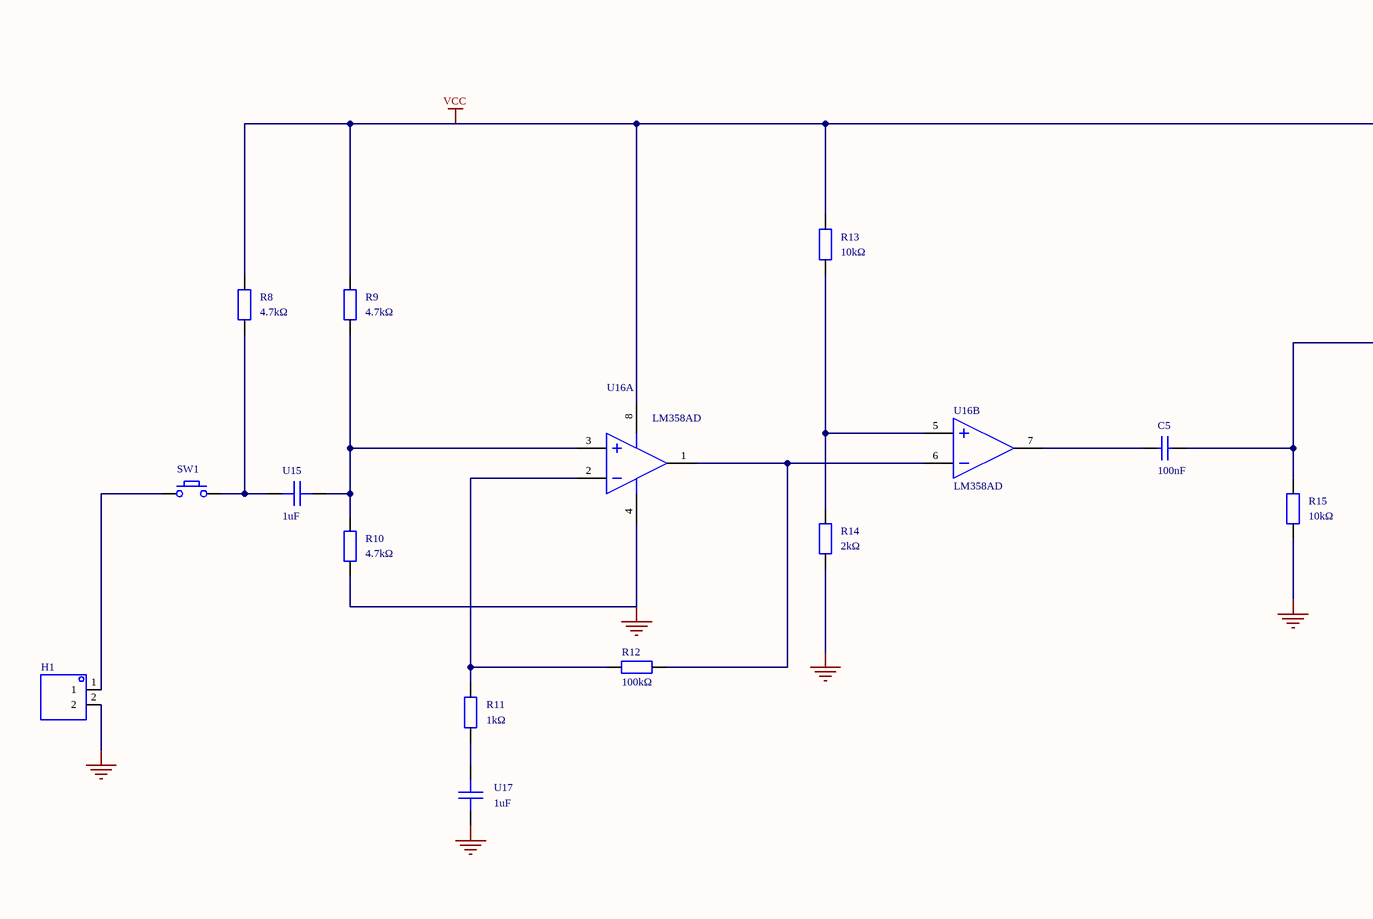
[diagram p0: MISC51104-3.schdoc, left]
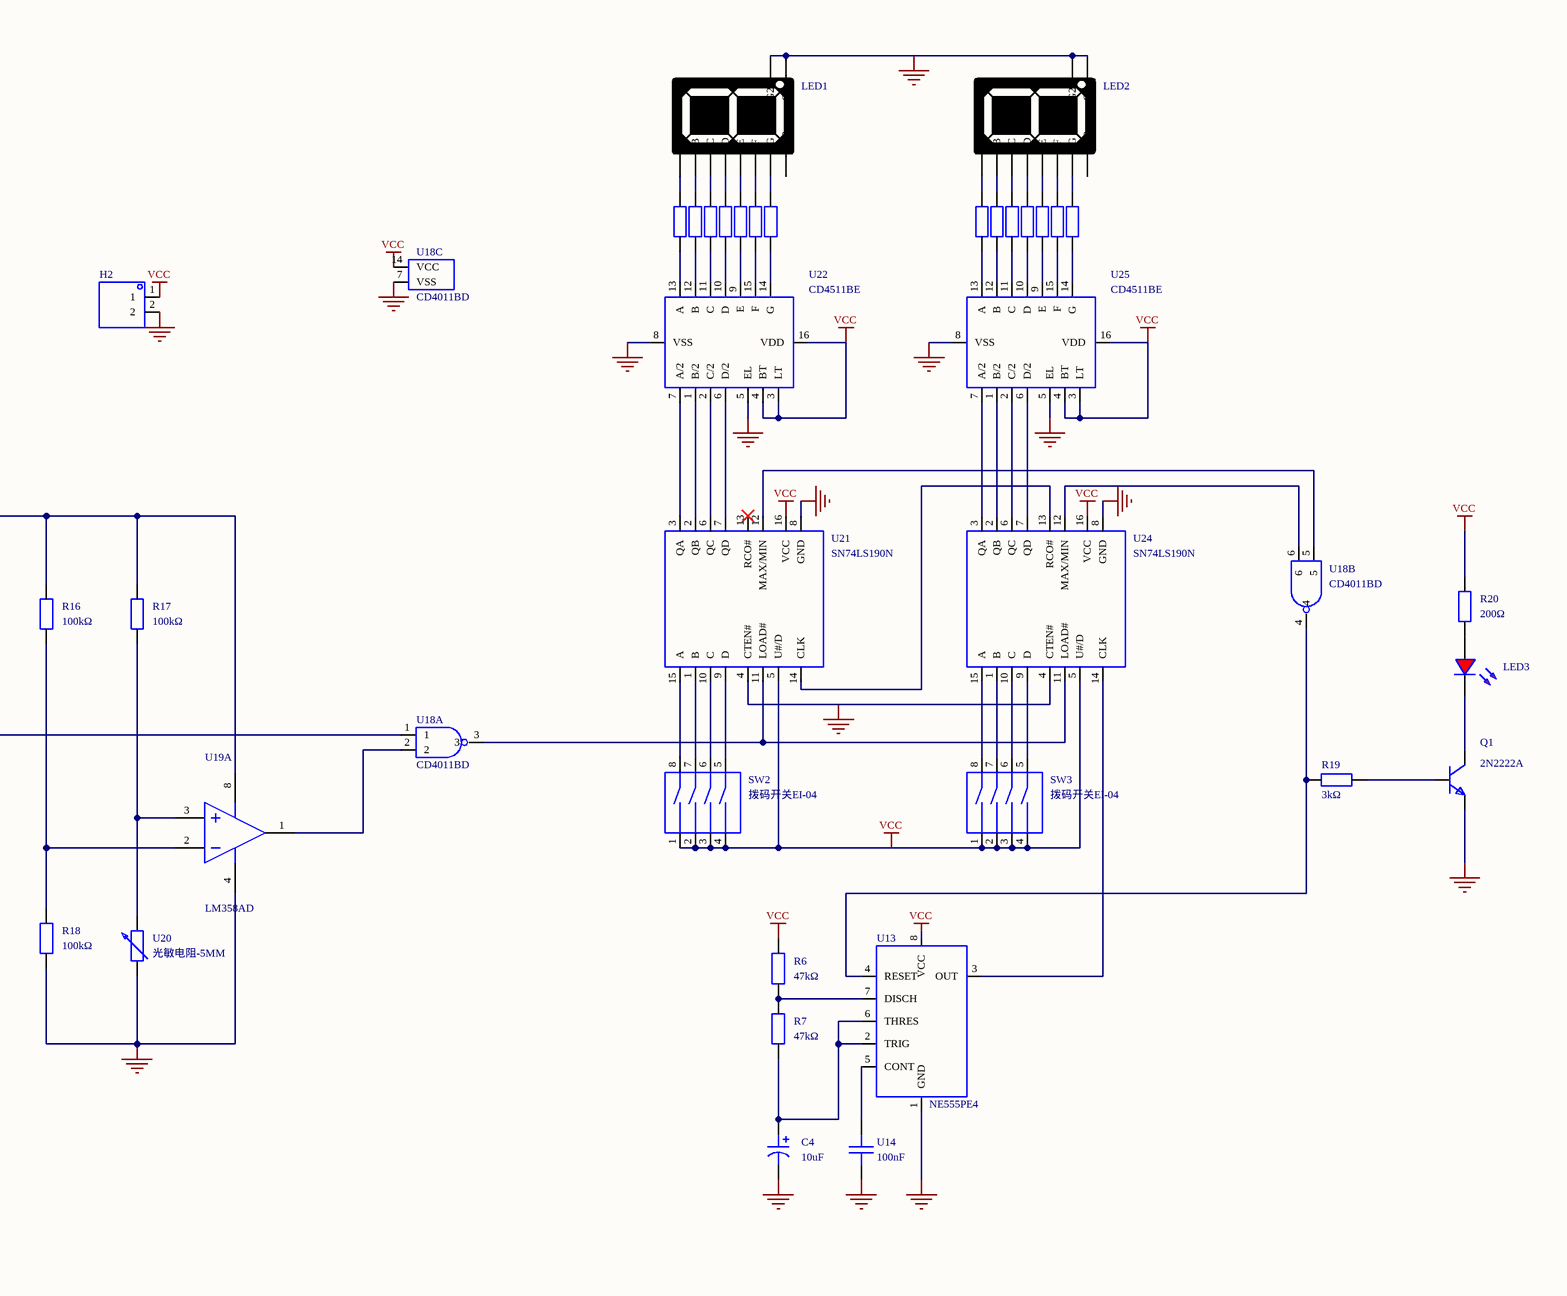
[diagram p1: MISC51104-3.schdoc, right]
# Altium project MISC51104-2.PrjPcb
1 sheet, 52 parts. Net scope: global (net labels, ports and power ports of the same name join across sheets).
Board file: MISC51104.pcbdoc

## Sheet MISC51104-3.schdoc
size 594 x 419 mm; Version: V1.0; @Project Name: MISC51104; @Page Count: 1; @Update Date: 2025-06-07; @Create Date: 2025-06-07; @Schematic Name: MISC51104; @Page No: 1; @Create Time: 21:33:00; @Update Time: 12:58:40; @Board Name: MISC51104

### Parts
C4  10uF  [CAP-TH_BD5.0-P2.00-D0.5-FD]
C5  100nF  [CAP-TH_L4.0-W2.5-P2.50-D0.5-A]
H1  (no value)  [HDR-TH_2P-P2.54-V-M-1]
H2  (no value)  [HDR-TH_2P-P2.54-V-M-1]
LED1  (no value)  [LED-SEG-TH_10P-L12.6-W19.0-P2.54-S15.24-BL]
LED2  (no value)  [LED-SEG-TH_10P-L12.6-W19.0-P2.54-S15.24-BL]
LED3  (no value)  [LED_TH-3mm]
Q1  2N2222A  [TO-92-3_L4.9-W3.7-P1.27-L]
R6  47kΩ  [Res_1/8W]
R7  47kΩ  [Res_1/8W]
R8  4.7kΩ  [Res_1/8W]
R9  4.7kΩ  [Res_1/8W]
R10  4.7kΩ  [Res_1/8W]
R11  1kΩ  [Res_1/8W]
R12  100kΩ  [Res_1/8W]
R13  10kΩ  [Res_1/8W]
R14  2kΩ  [Res_1/8W]
R15  10kΩ  [Res_1/8W]
R16  100kΩ  [Res_1/8W]
R17  100kΩ  [Res_1/8W]
R18  100kΩ  [Res_1/8W]
R19  3kΩ  [Res_1/8W]
R20  200Ω  [Res_1/8W]
R21  10kΩ  [Res_1/8W]  (value not drawn)
R22  10kΩ  [Res_1/8W]  (value not drawn)
R23  10kΩ  [Res_1/8W]  (value not drawn)
R24  10kΩ  [Res_1/8W]  (value not drawn)
R25  10kΩ  [Res_1/8W]  (value not drawn)
R26  10kΩ  [Res_1/8W]  (value not drawn)
R27  10kΩ  [Res_1/8W]  (value not drawn)
R28  10kΩ  [Res_1/8W]  (value not drawn)
R29  10kΩ  [Res_1/8W]  (value not drawn)
R30  10kΩ  [Res_1/8W]  (value not drawn)
R31  10kΩ  [Res_1/8W]  (value not drawn)
R32  10kΩ  [Res_1/8W]  (value not drawn)
R33  10kΩ  [Res_1/8W]  (value not drawn)
R34  10kΩ  [Res_1/8W]  (value not drawn)
SW1  (no value)  [Key_TH_3.5x6x4.3]
SW2  拨码开关EI-04  [SW-TH_DIPSWITCHEI-04]
SW3  拨码开关EI-04  [SW-TH_DIPSWITCHEI-04]
U13  NE555PE4  [PDIP-8_L9.6-W6.4-P2.54-LS7.9-BL-1]
U14  100nF  [CAP-TH_L4.5-W3.0-P2.50-D0.5]
U15  1uF  [CAP-TH_L4.0-W2.5-P2.50-D0.5]
U16  LM358AD  [SOP-8_L4.9-W3.9-P1.27-LS6.0-BL]  (parts A,B of 2)
U17  1uF  [CAP-TH_L4.0-W2.5-P2.50-D0.5]
U18  CD4011BD  [PDIP-14_L19.3-W6.4-P2.54-LS7.9-BL-1]  (parts A,B,C of 3)
U19  LM358AD  [SOP-8_L4.9-W3.9-P1.27-LS6.0-BL]  (part A of 2)
U20  光敏电阻-5MM  [RES-TH_L4.9-W4.3-P3.4]
U21  SN74LS190N  [PDIP-16_L19.2-W6.6-P2.54-LS7.6-BL]
U22  CD4511BE  [DIP-16_L19.8-W6.5-P2.54-LS7.6-BL]
U24  SN74LS190N  [PDIP-16_L19.2-W6.6-P2.54-LS7.6-BL]
U25  CD4511BE  [DIP-16_L19.8-W6.5-P2.54-LS7.6-BL]

### Nets
GND: C4.2 H1.2 H2.2 LED1.3(G1) LED1.8(G2) LED2.3(G1) LED2.8(G2) Q1.1(E) R10.1 R14.1 R15.1 R18.1 U13.1(GND) U14.1 U16.4(VEE) U17.1 U18.7(VSS) U19.4(VEE) U20.1 U21.4(CTEN#) U21.8(GND) U22.5(EL) U22.8(VSS) U24.4(CTEN#) U24.8(GND) U25.5(EL) U25.8(VSS)
VCC: H2.1 R6.2 R8.2 R9.2 R13.2 R16.2 R17.2 R20.2 SW2.1 SW2.2 SW2.3 SW2.4 SW3.1 SW3.2 SW3.3 SW3.4 U13.8(VCC) U16.8(VCC) U18.14(VCC) U19.8(VCC) U21.5(U#/D) U21.16(VCC) U22.3(LT) U22.4(BT) U22.16(VDD) U24.5(U#/D) U24.16(VCC) U25.3(LT) U25.4(BT) U25.16(VDD)
NetC4_1: C4.1 R7.1 U13.2(TRIG) U13.6(THRES)
NetC5_1: C5.1 U16.7(OUT2)
NetC5_2: C5.2 R15.2 U18.1
NetH1_1: H1.1 SW1.A
NetLED1_1: LED1.1(E) R25.2
NetLED1_2: LED1.2(D) R24.2
NetLED1_4: LED1.4(C) R23.2
NetLED1_6: LED1.6(B) R22.2
NetLED1_7: LED1.7(A) R21.2
NetLED1_9: LED1.9(F) R26.2
NetLED1_10: LED1.10(G) R27.2
NetLED2_1: LED2.1(E) R32.2
NetLED2_2: LED2.2(D) R31.2
NetLED2_4: LED2.4(C) R30.2
NetLED2_6: LED2.6(B) R29.2
NetLED2_7: LED2.7(A) R28.2
NetLED2_9: LED2.9(F) R33.2
NetLED2_10: LED2.10(G) R34.2
NetLED3_1: LED3.1(C) R20.1
NetLED3_2: LED3.2(A) Q1.3(C)
NetQ1_2: Q1.2(B) R19.1
NetR6_1: R6.1 R7.2 U13.7(DISCH)
NetR8_1: R8.1 SW1.B U15.1
NetR9_1: R9.1 R10.2 U15.2 U16.3(IN1-)
NetR11_1: R11.1 U17.2
NetR11_2: R11.2 R12.1 U16.2(IN1+)
NetR12_2: R12.2 U16.1(OUT1) U16.6(IN2-)
NetR13_1: R13.1 R14.2 U16.5(IN2+)
NetR16_1: R16.1 R18.2 U19.2(IN1+)
NetR17_1: R17.1 U19.3(IN1-) U20.2
NetR19_2: R19.2 U13.4(RESET) U18.4
NetR21_1: R21.1 U22.13(A)
NetR22_1: R22.1 U22.12(B)
NetR23_1: R23.1 U22.11(C)
NetR24_1: R24.1 U22.10(D)
NetR25_1: R25.1 U22.9(E)
NetR26_1: R26.1 U22.15(F)
NetR27_1: R27.1 U22.14(G)
NetR28_1: R28.1 U25.13(A)
NetR29_1: R29.1 U25.12(B)
NetR30_1: R30.1 U25.11(C)
NetR31_1: R31.1 U25.10(D)
NetR32_1: R32.1 U25.9(E)
NetR33_1: R33.1 U25.15(F)
NetR34_1: R34.1 U25.14(G)
NetSW2_5: SW2.5 U21.9(D)
NetSW2_6: SW2.6 U21.10(C)
NetSW2_7: SW2.7 U21.1(B)
NetSW2_8: SW2.8 U21.15(A)
NetSW3_5: SW3.5 U24.9(D)
NetSW3_6: SW3.6 U24.10(C)
NetSW3_7: SW3.7 U24.1(B)
NetSW3_8: SW3.8 U24.15(A)
NetU13_3: U13.3(OUT) U24.14(CLK)
NetU13_5: U13.5(CONT) U14.2
NetU18_2: U18.2 U19.1(OUT1)
NetU18_3: U18.3 U21.11(LOAD#) U24.11(LOAD#)
NetU18_5: U18.5 U21.12(MAX/MIN)
NetU18_6: U18.6 U24.12(MAX/MIN)
NetU21_2: U21.2(QB) U22.1(B/2)
NetU21_3: U21.3(QA) U22.7(A/2)
NetU21_6: U21.6(QC) U22.2(C/2)
NetU21_7: U21.7(QD) U22.6(D/2)
NetU21_14: U21.14(CLK) U24.13(RCO#)
NetU24_2: U24.2(QB) U25.1(B/2)
NetU24_3: U24.3(QA) U25.7(A/2)
NetU24_6: U24.6(QC) U25.2(C/2)
NetU24_7: U24.7(QD) U25.6(D/2)

Not connected (* = marked no-connect by the designer): LED1 5(DP); LED2 5(DP); U21 13(RCO#)*

### Notes on the sheet
- 2025-06-07
- 原理图
- P1
- 版本
- 尺寸
- A4
- 页    1    共    1

### Library data of the parts
C4 = SHG63V10UF03EC0822: 容值:10uF;精度:±20%;额定电压:63V;; AddInBom: yes; ModelId: aba3b94bdab6406eb4f45c9c765c730e; ModelTransform: 196.85,196.517,0,0,0,0,0,0,-196.85; Tolerance: ±20%; Voltage Rating: 63V; Symbol: SHG63V10UF03EC0822; Device: SHG63V10UF03EC0822; LCSC Part Name: 停产 10uF ±20% 63V; SupplierPart: C5263880; ManufacturerPart: SHG63V10UF03EC0822; Supplier Footprint: 插件,D5xL11mm; JLCPCB Part Class: 扩展库; Datasheet: https://atta.szlcsc.com/upload/public/pdf/source/20221206/74D9A2C5191757C58A566DD8357A6A8B.pdf; Supplier: LCSC; ConvertToPcb: yes; FootprintName: CAP-TH_BD5.0-P2.00-D0.5-FD; ModelName: CAP-TH_BD5.0-P2.00-D0.5-FD; Value: 10uF; Diameter: 5mm; Height - Seated (Max): 11mm
C5 = FA18X7R1H104KNU00: 容值:100nF;精度:±10%;额定电压:50V;温度系数:X7R;; Manufacturer: TDK; AddInBom: yes; ModelId: 286ce451e059442e92b487a621b9c1b6; ModelTransform: 217.63405,98.8187,0,0,0,0,0,0,-196.85; Tolerance: ±10%; Voltage Rated: 50V; Temperature Coefficient: X7R; Symbol: FA18X7R1H104KNU00; Device: FA18X7R1H104KNU00; LCSC Part Name: 100nF ±10% 50V; SupplierPart: C1622804; ManufacturerPart: FA18X7R1H104KNU00; Supplier Footprint: 插件; JLCPCB Part Class: 扩展库; Datasheet: https://atta.szlcsc.com/upload/public/pdf/source/20210607/0A2A90FBDDBAB681A19577D378B4B30C.pdf; Supplier: LCSC; ConvertToPcb: yes; FootprintName: CAP-TH_L4.0-W2.5-P2.50-D0.5-A; ModelName: CAP-TH_L4.0-W2.5-P2.50-D0.5-A; Value: 100nF
H1 H2 = HDR-M_2.54_1x2P: Symbol: 210S-1*2P L=11.6MMGold-plated black; ConvertToPcb: yes; ModelId: 79b2e9f2d70a4d68a1b7098f27c6d4c5; ModelName: HDR-M-2.54_1x2; ModelTransform: 200,100,0,0,0,0,0,0,-118.11; Device: HDR-M_2.54_1x2P; AddInBom: yes; SupplierPart: C124375; Supplier Footprint: 插件; FootprintName: HDR-TH_2P-P2.54-V-M-1
LED1 LED2 = LED_SEG_TH_0.56x1: Symbol: LED_SEG_TH_0.56*1; ConvertToPcb: yes; ModelId: 16c3aae6d39e4ecc9e744d6eeac8d57b; ModelName: LED-SEG-TH_0.56_1p; ModelTransform: 496.062,748.03,0,0,0,0,0,0,-137.795; Device: LED_SEG_TH_0.56x1; AddInBom: yes; Supplier Footprint: 插件; FootprintName: LED-SEG-TH_10P-L12.6-W19.0-P2.54-S15.24-BL
LED3 = LED_TH-R_3mm: ConvertToPcb: yes; ModelId: a497c992633541038a38947cdc58012f; ModelName: LED-TH-3mm_R; ModelTransform: 141.274,153.327,0,0,0,0,-5.984,0,-137.795; Symbol: LED_TH-R; Device: LED_TH-R_3mm; AddInBom: yes; FootprintName: LED_TH-3mm; Supplier Footprint: 插件
Q1 = 2N2222A: 晶体管类型:NPN;集电极电流(Ic):600mA;集射极击穿电压(Vceo):40V;功率(Pd):625mW;直流电流增益(hFE@Ic,Vce):40@500mA,10V;; Manufacturer: ST(先科); Symbol: 2N2222; AddInBom: yes; ModelId: db569d051dcd4484acf2f9e50678fca3; ModelTransform: 180.7872,141.4455,0,0,0,0,0,22.677,-196.85; Transistor Type: NPN; Collector Current (Ic): 600mA; Collector-Emitter Breakdown Voltage (Vceo): 40V; Power Dissipation (Pd): 625mW; Transition Frequency (fT): 250MHz; Collector Cut-Off Current (Icbo): 10nA; Collector-Emitter Saturation Voltage (VCE(sat)@Ic,Ib): 1V@500mA,50mA; Device: 2N2222A; LCSC Part Name: NPN 电流:600mA 耐压:40V; SupplierPart: C118536; ManufacturerPart: 2N2222A; Supplier Footprint: TO-92-3; Datasheet: https://atta.szlcsc.com/upload/public/pdf/source/20170719/C118536_1500457734789828244.pdf; Supplier: LCSC; ConvertToPcb: yes; FootprintName: TO-92-3_L4.9-W3.7-P1.27-L; ModelName: TO-92-3_L4.9-W3.7-P1.27-L; DC Current Gain (hFE@Ic,Vce): 40@500mA,10V; Operating Temperature: -
R6-R34 = Res_AXIAL-1/8W: ConvertToPcb: yes; SymbolName: 电阻; ModelId: b2b5ae7ae4c642178fe0039925c86a3f; ModelName: RES-TH_BD1.8-L3.2-P7.20-D0.4; ModelTransform: 282.86,66.88,253.09,0,0,0,0,0,-191; Device: Res_AXIAL-1/8W; AddInBom: yes; Supplier Footprint: 轴向引线; FootprintName: Res_1/8W
  R6 R7: Value: 47kΩ
  R8-R10: Value: 4.7kΩ
  R11: Value: 1kΩ
  R12 R16-R18: Value: 100kΩ
  R13 R15 R21-R34: Value: 10kΩ
  R14: Value: 2kΩ
  R19: Value: 3kΩ
  R20: Value: 200Ω
SW1 = Key_TH_3.5x6x4.3: ConvertToPcb: yes; ModelId: c3523f9014d949d7ba5445190a3178990819f05c4eef4c71ace90d822a990e87; ModelName: SW-TH_L6.0-W3.5-H5.0-P6.5; ModelTransform: 308.49,137.8,335.08,0,0,0,0,0,-129.92; Device: Key_TH_3.5x6x4.3; AddInBom: yes; Supplier Footprint: 插件; SymbolName: Key_TH_3.5x6x4.3; FootprintName: Key_TH_3.5x6x4.3
SW2 SW3 = 拨码开关EI-04: 类型:平拨,凸起式;电路结构:单刀单掷;开关位数:4位;使用寿命:-;颜色:黑色;; Manufacturer: 圜达; Symbol: DIP switchEI-04; AddInBom: yes; ModelId: 05004328256048a2b98ea2194ea80753; ModelName: SW-TH_DIPSWITCHEI-04-L10.1-W6.0-H3.4-P2.54-LS7.6; ModelTransform: 396.0622,309.842,0,0,0,0,0,0,-137.795; Circuit: 单刀单掷; Number of Positions: 4位; Device: 拨码开关EI-04; LCSC Part Name: 拨码开关EI-04; SupplierPart: C99987; ManufacturerPart: 拨码开关EI-04; Supplier Footprint: -; JLCPCB Part Class: 扩展库; Datasheet: https://atta.szlcsc.com/upload/public/pdf/source/20170504/1493892386551.pdf; Supplier: LCSC; ConvertToPcb: yes; FootprintName: SW-TH_DIPSWITCHEI-04; Type: 平拨,凸起式; Lead Pitch: 2.54mm; Operating Life: -; Color: 黑色
U13 = NE555PE4: 单精度计时器 8-PDIP 0 to 70; Manufacturer: TI(德州仪器); AddInBom: yes; ModelId: 1b8eaf096e7944deafe216467068c10e; ModelTransform: 377.952,318.897,0,0,0,0,0,0,-118.11; Symbol: NE555PE4; Device: NE555PE4; LCSC Part Name: NE555PE4; SupplierPart: C2859604; ManufacturerPart: NE555PE4; Supplier Footprint: PDIP-8; Datasheet: https://www.ti.com/cn/lit/gpn/sa555; Supplier: LCSC; ConvertToPcb: yes; FootprintName: PDIP-8_L9.6-W6.4-P2.54-LS7.9-BL-1; ModelName: PDIP-8_L9.6-W6.4-P2.54-LS7.9-BL-1
U14 = FA14X8R1H104KNU00: 容值:100nF;精度:±10%;额定电压:50V;温度系数:X8R;; Manufacturer: TDK; AddInBom: yes; ModelId: 4f3b11b509834e358e085933e775514f; ModelTransform: 217.61949,118.11,0,0,0,0,0,0,-196.85; Tolerance: ±10%; Voltage Rated: 50V; Temperature Coefficient: X8R; Symbol: FA14X8R1H104KNU00; Device: FA14X8R1H104KNU00; LCSC Part Name: 100nF ±10% 50V; SupplierPart: C1629759; ManufacturerPart: FA14X8R1H104KNU00; Supplier Footprint: 插件; JLCPCB Part Class: 扩展库; Datasheet: https://atta.szlcsc.com/upload/public/pdf/source/20210503/3ED621F3684B6FF62914AEB5593A787B.pdf; Supplier: LCSC; ConvertToPcb: yes; FootprintName: CAP-TH_L4.5-W3.0-P2.50-D0.5; ModelName: CAP-TH_L4.5-W3.0-P2.50-D0.5; Value: 100nF
U15 U17 = FA18X7R1E105KRU00: 容值:1uF;精度:±10%;额定电压:25V;温度系数:X7R;; Manufacturer: TDK; AddInBom: yes; ModelId: 29f34a7a495a447ab8bf96a7f673455e; ModelTransform: 189.7897,98.8187,0,0,0,0,0,0,-196.85; Tolerance: ±10%; Voltage Rated: 25V; Temperature Coefficient: X7R; Symbol: FA18X7R1E105KRU00; Device: FA18X7R1E105KRU00; LCSC Part Name: 1uF ±10% 25V; SupplierPart: C1632013; ManufacturerPart: FA18X7R1E105KRU00; Supplier Footprint: 插件; JLCPCB Part Class: 扩展库; Datasheet: https://atta.szlcsc.com/upload/public/pdf/source/20210607/0A2A90FBDDBAB681A19577D378B4B30C.pdf; Supplier: LCSC; ConvertToPcb: yes; FootprintName: CAP-TH_L4.0-W2.5-P2.50-D0.5; ModelName: CAP-TH_L4.0-W2.5-P2.50-D0.5; Value: 1uF
U16 U19 = LM358AD: 放大器数:双路;增益带宽积(GBP):1.1MHz;输入偏置电流(Ib):20nA;压摆率(SR):0.6V/us;; Manufacturer: ST(意法半导体); Relevance: []; AddInBom: yes; Number of Circuits: 双路; Gain Bandwidth Product(GBP): 1.1MHz; Current - Input Bias(Ib): 20nA; Output Current: 40mA; ModelId: 75c24a7891ee4dd6bdac16a7163ff87e; ModelName: SOP-8_L4.9-W3.9-P1.27-LS6.0-BL-1; ModelTransform: 192.913,236.22,0,0,0,0,0,0,0; Device: LM358AD; LCSC Part Name: LM358AD; SupplierPart: C5456123; ManufacturerPart: LM358AD; Supplier Footprint: SOIC-8; JLCPCB Part Class: 扩展库; Datasheet: https://atta.szlcsc.com/upload/public/pdf/source/20210324/C2649392_3AC2EBDF95F7F5F1B944475B4862C799.pdf; Supplier: LCSC; ConvertToPcb: yes; Slew Rate(SR): 0.6V/us; Operating Temperature: 0℃~+70℃; FootprintName: SOP-8_L4.9-W3.9-P1.27-LS6.0-BL
  U16: Symbol: LM358AD
  U19: SymbolName: LM358AD
U18 = CD4011BD: 逻辑类型:与非门;通道数:4;工作电压:3V~15V;; Manufacturer: Sungine(双竞集成); Relevance: []; AddInBom: yes; Logic Type: 与非门; Number of Channels: 4; Voltage - Supply: 3V~15V; ModelId: 850da569defe42bfb44bffbf61585822; ModelTransform: 751.967,309.842,0,0,0,0,0,0,-118.11; Device: CD4011BD; LCSC Part Name: CD4011BD; SupplierPart: C5274711; ManufacturerPart: CD4011BD; Supplier Footprint: DIP-14; JLCPCB Part Class: 扩展库; Datasheet: https://atta.szlcsc.com/upload/public/pdf/source/20221121/1C9119AF08500E1C210179F7AF6D460E.pdf; Supplier: LCSC; ConvertToPcb: yes; SymbolName: CD4011BD; FootprintName: PDIP-14_L19.3-W6.4-P2.54-LS7.9-BL-1; ModelName: PDIP-14_L19.3-W6.4-P2.54-LS7.9-BL-1
U20 = 光敏电阻-5MM: AddInBom: yes; ModelId: 8cda4899688949e78503a56fe341541c; ModelTransform: 169.291,200.6107,0,90,0,0,0,0,-196.85; Symbol: 光敏电阻-5MM; Device: 光敏电阻-5MM; LCSC Part Name: 光敏电阻-5MM; SupplierPart: C9900003115; ManufacturerPart: 光敏电阻-5MM; Supplier Footprint: RES-TH_4.3X4.9X3.37P; JLCPCB Part Class: 扩展库; Supplier: LCSC; ConvertToPcb: yes; FootprintName: RES-TH_L4.9-W4.3-P3.4; ModelName: RES-TH_L4.9-W4.3-P3.4
U21 U24 = SN74LS190N: AddInBom: yes; Symbol: SN74LS190N; Device: SN74LS190N; LCSC Part Name: SN74LS190N; SupplierPart: C9900109889; ManufacturerPart: SN74LS190N; Supplier Footprint: DIP-16; Supplier: LCSC; ConvertToPcb: yes; FootprintName: PDIP-16_L19.2-W6.6-P2.54-LS7.6-BL
U22 U25 = CD4511BE: CD4511B CMOS BCD 到 7 段 LED 锁存解码驱动器; Manufacturer: TI(德州仪器); AddInBom: yes; ModelId: 1d8537d07c784a01867ee00a159e9dcc; ModelName: DIP-16_L20.0-W6.4-H3.5-LS7.62-P2.54; ModelTransform: 787.4,311.8104,0,0,0,0,-0.003,0.001,-118.11; Symbol: CD4511BE; Device: CD4511BE; LCSC Part Name: CD4511BE; SupplierPart: C5327; ManufacturerPart: CD4511BE; Supplier Footprint: DIP-16; JLCPCB Part Class: 扩展库; Datasheet: https://www.ti.com/cn/lit/gpn/cd4511b; Supplier: LCSC; ConvertToPcb: yes; FootprintName: DIP-16_L19.8-W6.5-P2.54-LS7.6-BL